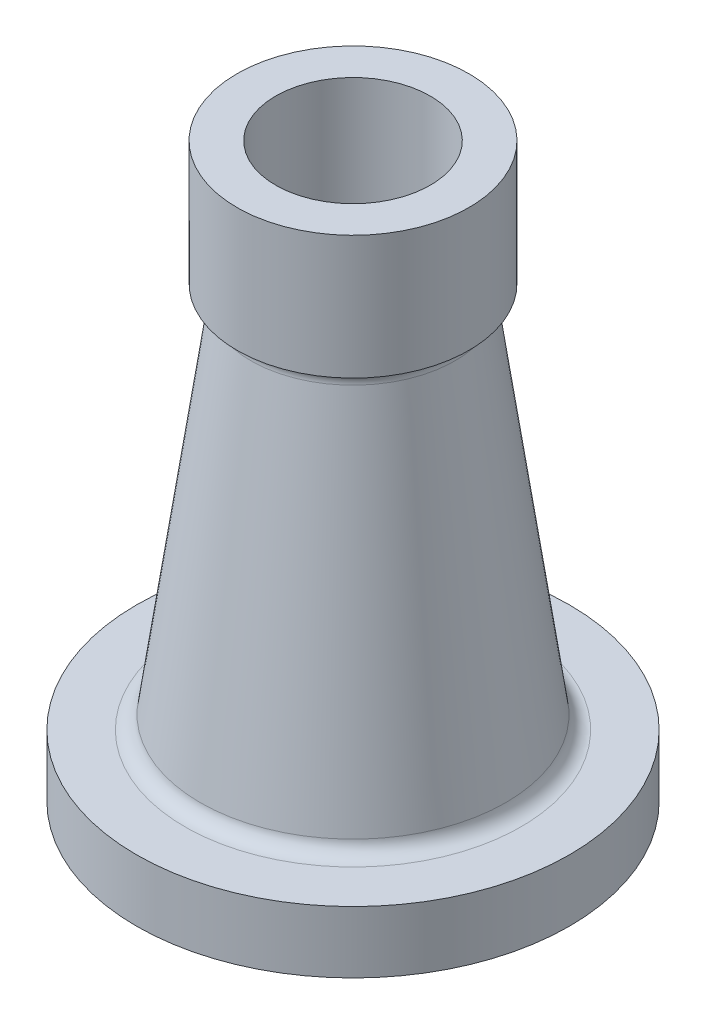
SolidWorks part; units mm, degrees
material "Chromium Copper, UNS C18200"
ref_plane "Front Plane" through (0, 0, 0) normal (0, 0, 1) x (1, 0, 0)
ref_plane "Top Plane" through (0, 0, 0) normal (0, 1, 0) x (1, 0, 0)
ref_plane "Right Plane" through (0, 0, 0) normal (1, 0, 0) x (0, 0, -1)
sketch "Sketch1" plane through (0, 0, 0) normal (0, 0, 1) x (1, 0, 0)
  line L0 (0, 92.5) -> (0, -92.5) construction
  line L1 (37.5, 92.5) -> (25, 92.5)
  line L2 (25, 92.5) -> (25, 25.7004)
  line L3 (37.5, 92.5) -> (37.5, 52.5)
  line L4 (70, -92.5) -> (50, -92.5)
  line L5 (70, -92.5) -> (70, -72.5)
  line L6 (70, -72.5) -> (54.3425, -72.5)
  line L7 (37.5, 52.5) -> (37.5, 48) construction
  line L8 (49.3918, -68.2003) -> (33.0444, 47.3697)
  line L9 (50, -92.5) -> (50, -89.5)
  line L10 (50, -89.5) -> (41.2952, -89.5)
  line L11 (41.2952, -89.5) -> (25, 25.7004)
  line L12 (38.5002, -69.7409) -> (22.1528, 45.8291) construction
  arc A0 (37.5, 52.5) -> (33.0444, 47.3697) centre (37.5, 48) ccw
  arc A1 (54.3425, -72.5) -> (49.3918, -68.2003) centre (54.3425, -67.5) cw
  point P15 (50, -72.5)
  dimension "D8" = 5
  dimension "D1" = 185
  dimension "D2" = 50
  dimension "D3" = 75
  dimension "D4" = 40
  dimension "D5" = 20
  dimension "20" = 20
  dimension "D6" = 20
  dimension "D7" = 4.5
  dimension "D9" = 140
  dimension "D10" = 3
  dimension "D11" = 11
revolve "Revolve1" add sketch "Sketch1" angle 360 about L0
